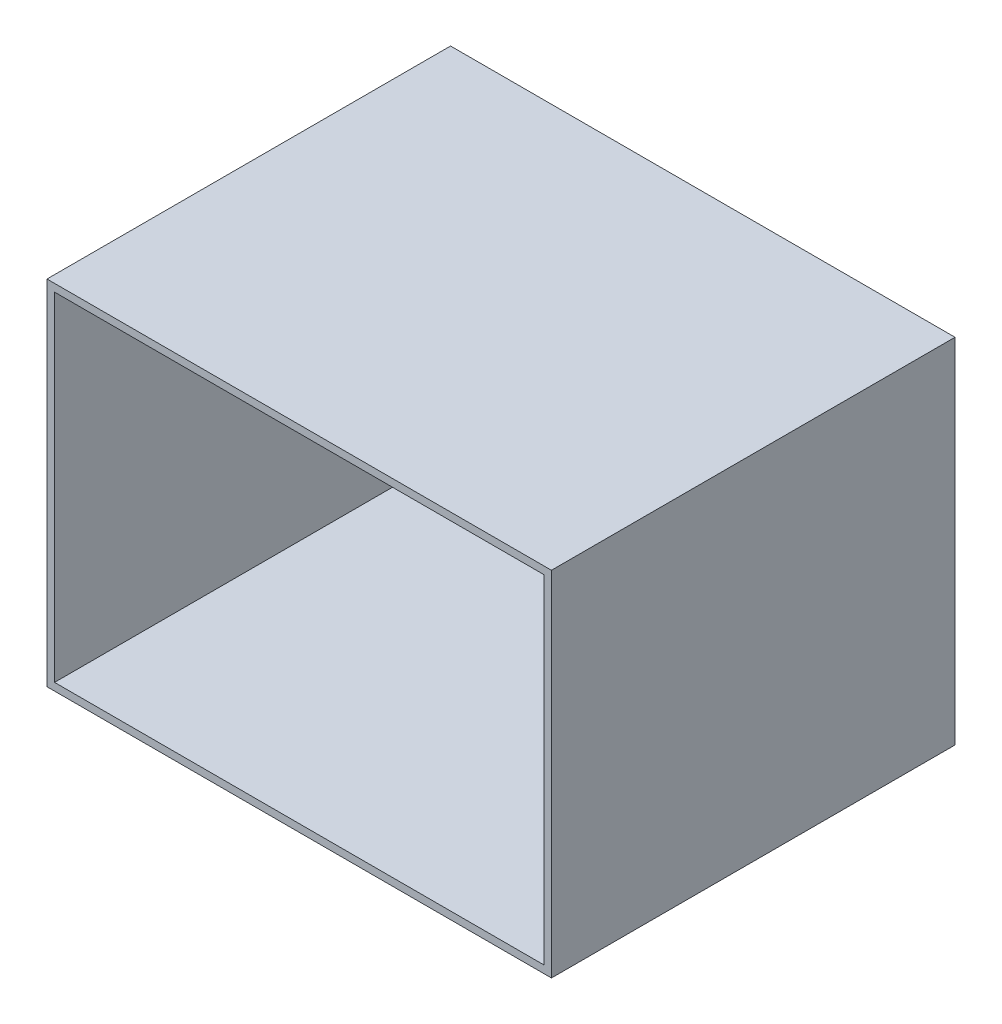
from build123d import *

# Parameters (mm, degrees)
SKETCH_1_W      = 200
SKETCH_1_H      = 140
SKETCH_1_W_2    = 194
SKETCH_1_H_2    = 134
EXTRUDE_1_DEPTH = 80


with BuildPart() as part:
    # 草图1 → 凸台-拉伸1 (new, symmetric)
    with BuildSketch(Plane.XY):
        Rectangle(SKETCH_1_W, SKETCH_1_H)
        Rectangle(SKETCH_1_W_2, SKETCH_1_H_2, mode=Mode.SUBTRACT)
    extrude(amount=EXTRUDE_1_DEPTH, both=True)


solid = part.part
